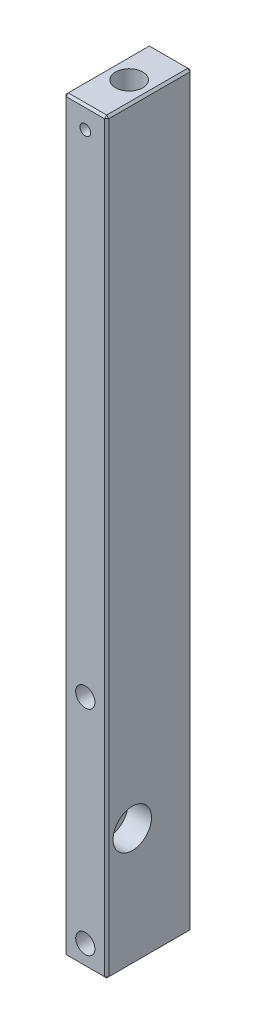
from build123d import *

# Parameters (mm, degrees)
SKETCH_1_W                = 20
SKETCH_1_H                = 40
EXTRUDE_1_DEPTH           = 350
SKETCH_2_R                = 6.4
CUT_EXTRUDE_1_DEPTH       = 20
HOLE_WIZARD_M6_1_D        = 5
CHAMFER_1_SIZE            = 1
HOLE_WIZARD_1_D           = 9
HOLE_WIZARD_1_CBORE_D     = 15
HOLE_WIZARD_1_CBORE_DEPTH = 9
HOLE_WIZARD_2_D           = 11
HOLE_WIZARD_2_DEPTH       = 50
HOLE_WIZARD_2_CBORE_D     = 18
HOLE_WIZARD_2_CBORE_DEPTH = 11
HOLE_WIZARD_2_TIP         = 3.304733405


with BuildPart() as part:
    # 草图1 → 凸台-拉伸1 (new body)
    with BuildSketch(Plane(origin=(0, 0, 0), x_dir=(1, 0, 0), z_dir=(0, 1, 0))):
        Rectangle(SKETCH_1_W, SKETCH_1_H)
    extrude(amount=EXTRUDE_1_DEPTH)

    # 草图2 → 切除-拉伸1 (cut)
    with BuildSketch(Plane(origin=(0, 350, 0), x_dir=(1, 0, 0), z_dir=(0, 1, 0))):
        with Locations(Location((0, 0.52, 0), (0, 0, 270))):
            Circle(SKETCH_2_R)
    extrude(amount=-CUT_EXTRUDE_1_DEPTH, mode=Mode.SUBTRACT)

    # M6 螺纹孔1 (through all)
    with Locations(Plane(origin=(0, 0, -20), x_dir=(-1, 0, 0), z_dir=(0, 0, -1))):
        with Locations((0, 340)):
            Hole(HOLE_WIZARD_M6_1_D / 2)

    # 倒角1
    chamfer_1_edges = [part.edges().sort_by_distance(p)[0] for p in [
        (-10, 350, 0),
        (0, 350, 20),
        (10, 350, 0),
        (0, 0, 20),
        (-10, 0, 0),
        (0, 0, -20),
        (10, 0, 0),
        (0, 350, -20),
        (10, 175, 20),
        (-10, 175, 20),
        (-10, 175, -20),
        (10, 175, -20),
    ]]
    chamfer(chamfer_1_edges, length=CHAMFER_1_SIZE)

    # 打孔尺寸(%根据)内六角圆柱头螺钉的类型1 (through all)
    with Locations(Plane(origin=(0, 0, -20), x_dir=(-1, 0, 0), z_dir=(0, 0, -1))):
        with Locations((0, 10), (0, 110)):
            CounterBoreHole(HOLE_WIZARD_1_D / 2, HOLE_WIZARD_1_CBORE_D / 2, HOLE_WIZARD_1_CBORE_DEPTH)

    # 打孔尺寸(%根据)内六角圆柱头螺钉的类型2
    with Locations(Plane(origin=(10, 0, 0), x_dir=(0, 0, -1), z_dir=(1, 0, 0))):
        with Locations((-8, 55.662088154)):
            CounterBoreHole(HOLE_WIZARD_2_D / 2, HOLE_WIZARD_2_CBORE_D / 2, HOLE_WIZARD_2_CBORE_DEPTH, depth=HOLE_WIZARD_2_DEPTH)
            with Locations((0, 0, -(HOLE_WIZARD_2_DEPTH + HOLE_WIZARD_2_TIP / 2))):  # 118° drill point
                Cone(0, HOLE_WIZARD_2_D / 2, HOLE_WIZARD_2_TIP, mode=Mode.SUBTRACT)


solid = part.part
